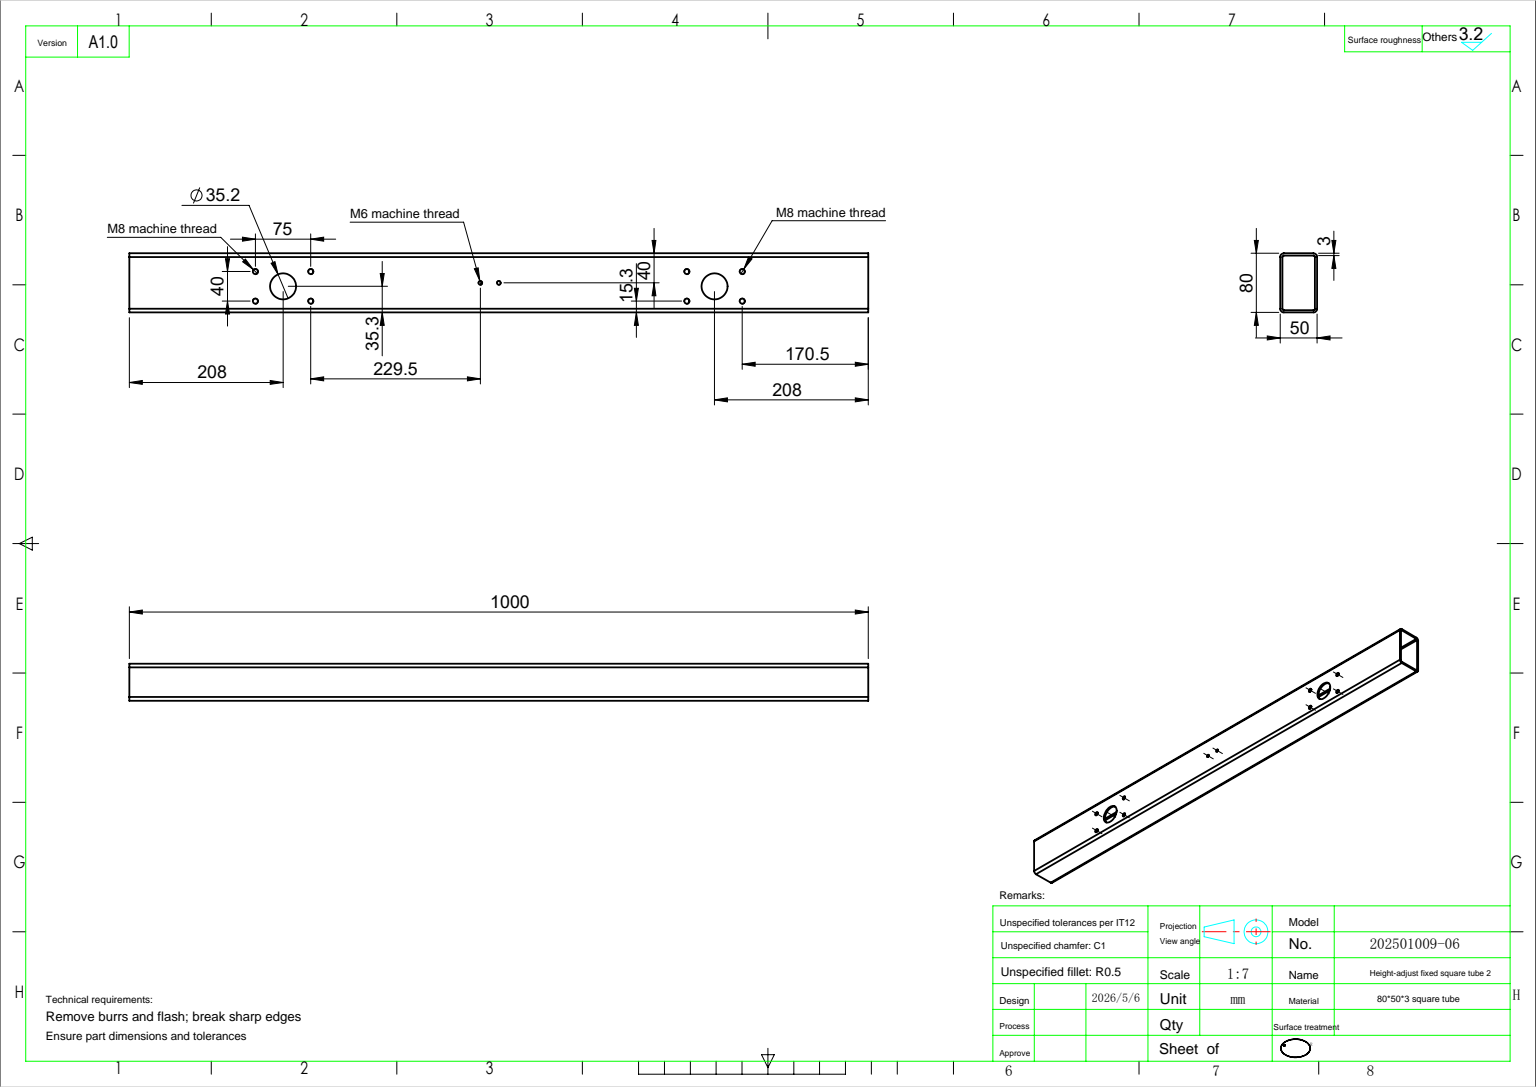
SolidWorks part; units mm, degrees
ref_plane "前视基准面" through (0, 0, 0) normal (0, 0, 1) x (1, 0, 0)
ref_plane "上视基准面" through (0, 0, 0) normal (0, 1, 0) x (1, 0, 0)
ref_plane "右视基准面" through (0, 0, 0) normal (1, 0, 0) x (0, 0, -1)
sketch "草图1" plane through (0, 0, 0) normal (0, 0, 1) x (1, 0, 0)
  line L1 (-40, 25) -> (40, 25)
  line L2 (-40, 25) -> (-40, -25)
  line L3 (-40, -25) -> (40, -25)
  line L4 (40, 25) -> (40, -25)
  line L5 (0, -25) -> (0, 25) construction
  line L6 (-40, 0) -> (40, 0) construction
  point P0 (0, 0)
  dimension "D1" = 50
  dimension "D2" = 80
extrude "凸台-拉伸1" add sketch "草图1" along normal blind 1000
fillet "圆角1" radius 5 4 edges at (40, -25, 500) (-40, -25, 500) (-40, 25, 500) (40, 25, 500)
shell "抽壳1" thickness 3
sketch "草图2" plane through (0, 25, 0) normal (0, 1, 0) x (1, 0, 0)
  line L0 (35, 0) -> (-35, 0) construction
  line L1 (40, 0) -> (40, -1000) construction
  circle A0 centre (-4.7, -208) radius 17.6
  circle A1 centre (-4.7, -792) radius 17.6
  dimension "D1" = 35.2
  dimension "D2" = 584
  dimension "D3" = 208
  dimension "D4" = 44.7
extrude "切除-拉伸1" cut sketch "草图2" against normal through all
sketch "草图3" plane through (0, 25, 0) normal (0, 1, 0) x (1, 0, 0)
  line L1 (-40, -1000) -> (-40, 0) construction
  line L2 (-4.7, -792) -> (56.5691, -792) construction
  line L4 (-4.7, -792) -> (-4.7, -1022.8371) construction
  line L5 (-4.7, -208) -> (56.5691, -208) construction
  line L6 (-4.7, -208) -> (-4.7, -299.499) construction
  circle A0 centre (15.3, -170.5) radius 3.4
  circle A1 centre (-24.7, -170.5) radius 3.4
  circle A2 centre (-24.7, -245.5) radius 3.4
  circle A3 centre (15.3, -245.5) radius 3.4
  circle A4 centre (15.3, -754.5) radius 3.4
  circle A5 centre (-24.7, -754.5) radius 3.4
  circle A6 centre (-24.7, -829.5) radius 3.4
  circle A7 centre (15.3, -829.5) radius 3.4
  point P23 (0, 0)
  point P25 (0, 0)
  dimension "D1" = 6.8
  dimension "D2" = 40
  dimension "D3" = 75
  dimension "D4" = 75
  dimension "D5" = 40
  dimension "D7" = 15.3
  dimension "D9" = 15.3
extrude "切除-拉伸2" cut sketch "草图3" against normal blind 10
cosmetic thread "装饰螺纹线1" parameters "D2"=8
cosmetic thread "装饰螺纹线2" parameters "D2"=8
cosmetic thread "装饰螺纹线3" parameters "D2"=8
cosmetic thread "装饰螺纹线4" parameters "D2"=8
cosmetic thread "装饰螺纹线5" parameters "D2"=8
cosmetic thread "装饰螺纹线6" parameters "D2"=8
cosmetic thread "装饰螺纹线7" parameters "D2"=8
cosmetic thread "装饰螺纹线8" parameters "D2"=8
sketch "草图4" plane through (0, 25, 0) normal (0, 1, 0) x (1, 0, 0)
  line L3 (35, -1000) -> (-35, -1000) construction
  line L4 (40, 0) -> (40, -1000) construction
  circle A0 centre (0, -475) radius 2.5
  circle A1 centre (0, -500) radius 2.5
  dimension "D1" = 5
  dimension "D3" = 25
  dimension "D2" = 40
  dimension "D4" = 500
extrude "切除-拉伸3" cut sketch "草图4" against normal blind 10
cosmetic thread "装饰螺纹线9"
cosmetic thread "装饰螺纹线10"
